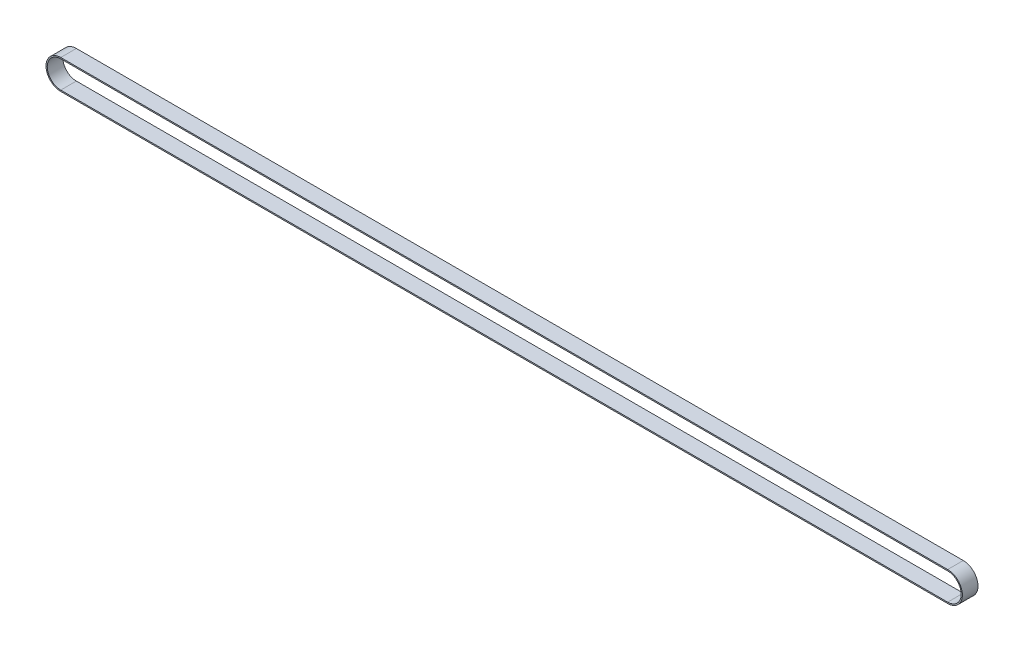
from build123d import *

# Parameters (mm, degrees)
EXTRUDE_1_DEPTH = 7.5


with BuildPart() as part:
    # 草图1 → 凸台-拉伸1 (new, symmetric)
    with BuildSketch(Plane.XY):
        with BuildLine():
            Line((0, 14.17), (852.5, 14.17))
            ThreePointArc((852.5, 14.17), (866.67, 0), (852.5, -14.17))
            Line((852.5, -14.17), (0, -14.17))
            ThreePointArc((0, -14.17), (-14.17, 0), (0, 14.17))
        make_face()
        with BuildLine():
            Line((0, 12.99), (852.5, 12.99))
            ThreePointArc((852.5, 12.99), (865.49, 0), (852.5, -12.99))
            Line((852.5, -12.99), (0, -12.99))
            ThreePointArc((0, -12.99), (-12.99, 0), (0, 12.99))
        make_face(mode=Mode.SUBTRACT)
    extrude(amount=EXTRUDE_1_DEPTH, both=True)


solid = part.part
